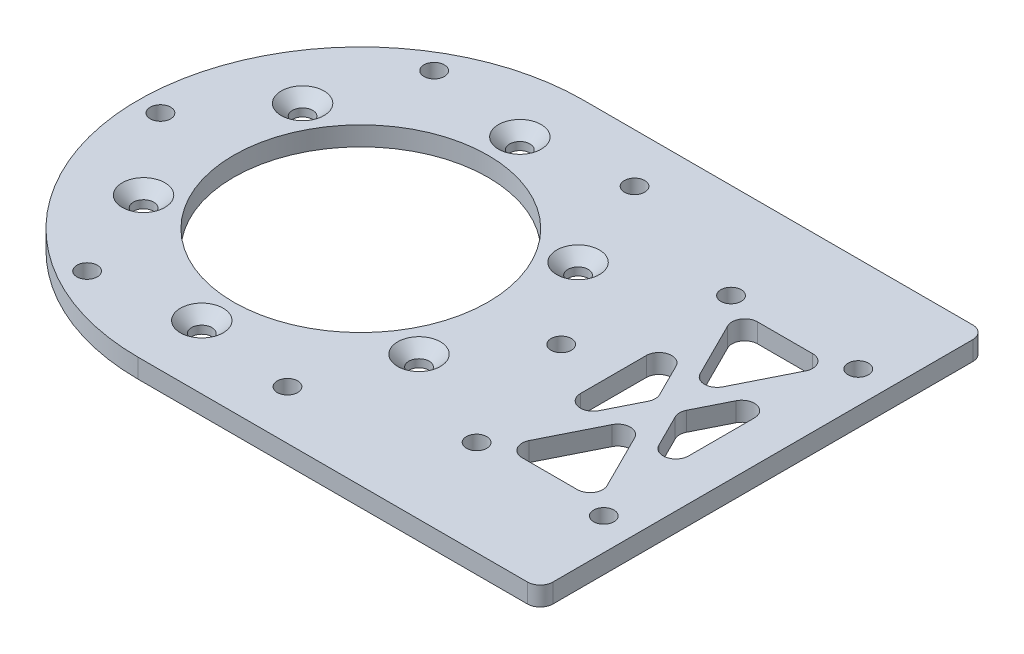
SolidWorks part; units mm, degrees
material "哈碳纤"
ref_plane "前视基准面" through (0, 0, 0) normal (0, 0, 1) x (1, 0, 0)
ref_plane "上视基准面" through (0, 0, 0) normal (0, 1, 0) x (1, 0, 0)
ref_plane "右视基准面" through (0, 0, 0) normal (1, 0, 0) x (0, 0, -1)
other "Configuration Table"
sketch "草图1" plane through (0, 0, 0) normal (0, 1, 0) x (1, 0, 0)
  line L1 (-63.2, 35) -> (0, 35)
  line L2 (-63.2, -35) -> (0, -35)
  line L3 (0, 35) -> (0, -35)
  line L4 (-25, 20) -> (-5, -20) construction
  line L5 (-25, -20) -> (-5, -20) construction
  line L6 (-25, -20) -> (-25, 20) construction
  line L7 (-25, 20) -> (-5, 20) construction
  line L8 (-5, -20) -> (-5, 20) construction
  arc A0 (-63.2, 35) -> (-63.2, -35) centre (-63.2, 0) ccw
  circle A2 centre (-63.2, 0) radius 25 construction
  circle A3 centre (-63.2, 25) radius 1.6
  circle A4 centre (-41.5494, 12.5) radius 1.6
  circle A5 centre (-41.5494, -12.5) radius 1.6
  circle A6 centre (-63.2, -25) radius 1.6
  circle A7 centre (-84.8506, -12.5) radius 1.6
  circle A8 centre (-84.8506, 12.5) radius 1.6
  circle A9 centre (-63.2, 0) radius 20
  circle A10 centre (-25, 20) radius 1.6
  circle A11 centre (-5, 20) radius 1.6
  circle A12 centre (-5, -20) radius 1.6
  circle A13 centre (-25, -20) radius 1.6
  point P1 (-15, 0)
  point P2 (0, 0)
  point P26 (0, 0)
  dimension "D1" = 70
  dimension "D3" = 50
  dimension "D4" = 3.2
  dimension "D6" = 40
  dimension "D9" = 3.2
  dimension "D2" = 48.2
  dimension "D7" = 40
  dimension "D8" = 20
  dimension "D10" = 15
  dimension "D5" = 6
extrude "凸台-拉伸1" add sketch "草图1" along normal blind 3
hole_wizard "M3 六角凹锥坑螺钉的锥形沉头孔1" positions "3D草图1" profile "草图2" countersink size "M3" standard "ISO" end condition through all
sketch3d "3D草图1"
  line L0 (-63.2, 3, -25) -> (-63.2, 0, -25) construction
  line L1 (-41.5494, 3, -12.5) -> (-41.5494, 0, -12.5) construction
  line L2 (-41.5494, 3, 12.5) -> (-41.5494, 0, 12.5) construction
  line L3 (-63.2, 3, 25) -> (-63.2, 0, 25) construction
  line L4 (-84.8506, 3, 12.5) -> (-84.8506, 0, 12.5) construction
  line L5 (-84.8506, 3, -12.5) -> (-84.8506, 0, -12.5) construction
  point P0 (-63.2, 3, -25)
  point P4 (-41.5494, 3, -12.5)
  point P8 (-41.5494, 3, 12.5)
  point P12 (-63.2, 3, 25)
  point P16 (-84.8506, 3, 12.5)
  point P20 (-84.8506, 3, -12.5)
sketch "草图2" plane through (-63.2, 3, -25) normal (1, 0, 0) x (0, 0, 1)
  line L0 (0, 0) -> (0, 3)
  line L1 (0, 3) -> (1.6, 3)
  line L2 (1.6, 3) -> (1.6, 1.76)
  line L3 (1.6, 1.76) -> (3.36, 0)
  line L5 (3.36, 0) -> (0, 0)
  line L6 (-1.6, 1.76) -> (-3.36, 0) construction
  line L11 (0, -6.35) -> (0, 107.95) construction
  dimension "通孔孔直径" = 3.2
  dimension "通孔孔深度" = 3
  dimension "近端锥形沉头孔直径" = 6.72
  dimension "近端锥形沉头孔角度" = 90
sketch "草图3" plane through (0, 3, 0) normal (0, 1, 0) x (1, 0, 0)
  circle A0 centre (-63.2, 0) radius 31.5 construction
  circle A1 centre (-31.7, 0) radius 1.6
  circle A2 centre (-47.45, -27.2798) radius 1.6
  circle A3 centre (-78.95, -27.2798) radius 1.6
  circle A4 centre (-94.7, 0) radius 1.6
  circle A5 centre (-78.95, 27.2798) radius 1.6
  circle A6 centre (-47.45, 27.2798) radius 1.6
  dimension "D1" = 63
  dimension "D2" = 3.2
  dimension "D3" = 6
extrude "切除-拉伸1" cut sketch "草图3" against normal blind 10
sketch "草图4" plane through (0, 3, 0) normal (0, 1, 0) x (1, 0, 0)
  line L0 (-25, -21.5) -> (-5, -21.5)
  line L1 (-25, -20) -> (-5, -20)
  line L2 (-25, -20) -> (-25, 20)
  line L3 (-25, 20) -> (-5, 20)
  line L4 (-5, -20) -> (-5, 20)
  line L5 (-25, -20) -> (-5, 20)
  line L6 (-25, 20) -> (-5, -20)
  line L7 (-23.5, -20) -> (-23.5, 20)
  line L8 (-25, 18.5) -> (-5, 18.5)
  line L9 (-3.5, -20) -> (-3.5, 20)
  line L10 (-23.6584, -20.6708) -> (-3.6584, 19.3292)
  line L11 (-26.3416, 19.3292) -> (-6.3416, -20.6708)
  line L12 (-25, -18.5) -> (-5, -18.5)
  line L13 (-26.5, -20) -> (-26.5, 20)
  line L14 (-25, 21.5) -> (-5, 21.5)
  line L15 (-6.5, -20) -> (-6.5, 20)
  line L16 (-26.3416, -19.3292) -> (-6.3416, 20.6708)
  line L17 (-23.6584, 20.6708) -> (-3.6584, -19.3292)
  arc A0 (-25, -21.5) -> (-25, -18.5) centre (-25, -20) cw
  arc A1 (-5, -21.5) -> (-5, -18.5) centre (-5, -20) ccw
  arc A2 (-23.5, -20) -> (-26.5, -20) centre (-25, -20) cw
  arc A3 (-23.5, 20) -> (-26.5, 20) centre (-25, 20) ccw
  arc A4 (-25, 18.5) -> (-25, 21.5) centre (-25, 20) cw
  arc A5 (-5, 18.5) -> (-5, 21.5) centre (-5, 20) ccw
  arc A6 (-3.5, -20) -> (-6.5, -20) centre (-5, -20) cw
  arc A7 (-3.5, 20) -> (-6.5, 20) centre (-5, 20) ccw
  arc A8 (-23.6584, -20.6708) -> (-26.3416, -19.3292) centre (-25, -20) cw
  arc A9 (-3.6584, 19.3292) -> (-6.3416, 20.6708) centre (-5, 20) ccw
  arc A10 (-26.3416, 19.3292) -> (-23.6584, 20.6708) centre (-25, 20) cw
  arc A11 (-6.3416, -20.6708) -> (-3.6584, -19.3292) centre (-5, -20) ccw
  point P0 (-15, 0)
  point P5 (-25, -20)
  dimension "D1" = 1.5
  dimension "D2" = 1.5
extrude "切除-拉伸2" cut sketch "草图4" against normal blind 10 contours L7 L16 L11 | L10 L12 L11 | L8 L17 L16 | L10 L17 L15
fillet "圆角1" radius 2 14 edges at (-15, 1.5, 3.3541) (-7.4271, 1.5, 18.5) (-22.5729, 1.5, 18.5) (-6.5, 1.5, -13.6459) (-6.5, 1.5, 13.6459) (-13.3229, 1.5, 0) (0, 1.5, 35) (0, 1.5, -35) (-16.6771, 1.5, 0) (-23.5, 1.5, 13.6459) (-7.4271, 1.5, -18.5) (-15, 1.5, -3.3541) (-22.5729, 1.5, -18.5) (-23.5, 1.5, -13.6459)
